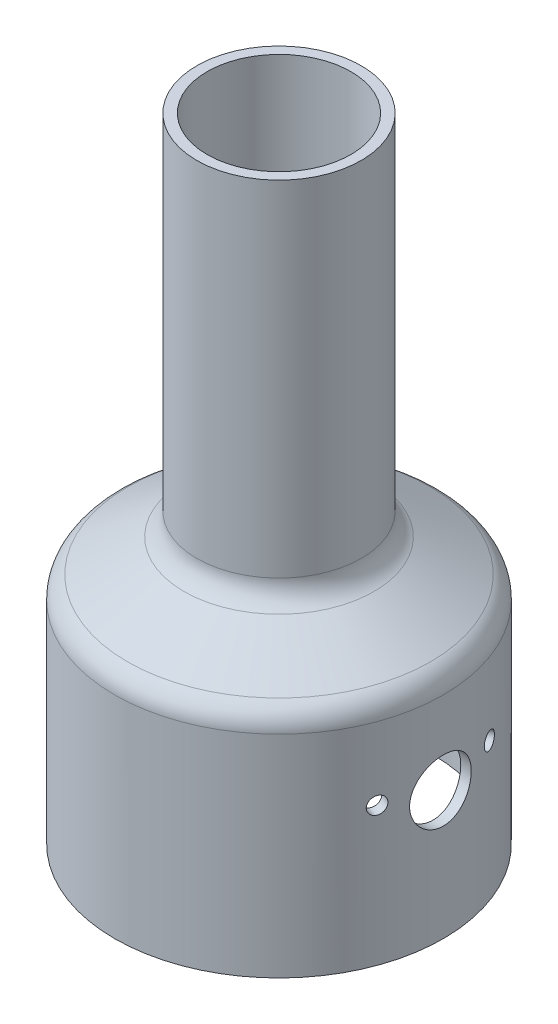
from build123d import *

# Parameters (mm, degrees)
FILLET1_R                       = 5
SHELL1_T                        = -2
CUT_EXTRUDE1_DEPTH              = 132.284070659
CUT_EXTRUDE1_DEPTH_BACK         = 132.284070659
SKETCH6_R                       = 6
M4_TAPPED_HOLE1_D               = 3.3
M4_TAPPED_HOLE1_DEPTH           = 10.1
M4_TAPPED_HOLE1_TIP             = 0.991420021
M4_TAPPED_HOLE1_ON_FACE_2_D     = 3.3
M4_TAPPED_HOLE1_ON_FACE_2_DEPTH = 10.1
M4_TAPPED_HOLE1_ON_FACE_2_TIP   = 0.991420021
M4_TAPPED_HOLE1_ON_FACE_3_D     = 3.3
M4_TAPPED_HOLE1_ON_FACE_3_DEPTH = 10.1
M4_TAPPED_HOLE1_ON_FACE_3_TIP   = 0.991420021
M4_TAPPED_HOLE1_ON_FACE_4_D     = 3.3
M4_TAPPED_HOLE1_ON_FACE_4_DEPTH = 10.1
M4_TAPPED_HOLE1_ON_FACE_4_TIP   = 0.991420021


with BuildPart() as part:
    # Sketch1 → Revolve1 (revolve)
    with BuildSketch(Plane.XY, mode=Mode.PRIVATE) as revolve1_sk:
        Polygon((0, 0), (-32, 0), (-32, 44), (-16, 53.237604307), (-16, 123.237604307), (0, 123.237604307), align=None)
    revolve(revolve1_sk.sketch.rotate(Axis((0, 123.237604307, 0), (0, -1, 0)), 270), axis=Axis((0, 123.237604307, 0), (0, -1, 0)))

    # Fillet1
    fillet1_edges = [part.edges().sort_by_distance(p)[0] for p in [
        (0, 53.237604307, -16),
        (0, 44, -32),
    ]]
    fillet(fillet1_edges, radius=FILLET1_R)

    # Shell1
    shell1_openings = [part.faces().sort_by_distance(p)[0] for p in [
        (0, 123.237604307, 0),
        (0, 0, 0),
    ]]
    offset(amount=SHELL1_T, openings=shell1_openings, kind=Kind.INTERSECTION)

    # Sketch6 → Cut-Extrude1 (cut, two sides: drawn at the far end of the back side and taken through both)
    with BuildSketch(Plane(origin=(0, 0, 0), x_dir=(0, 0, -1), z_dir=(1, 0, 0)).offset(-CUT_EXTRUDE1_DEPTH_BACK)):
        with Locations((0, 25)):
            Circle(SKETCH6_R)
    extrude(amount=CUT_EXTRUDE1_DEPTH + CUT_EXTRUDE1_DEPTH_BACK, mode=Mode.SUBTRACT)

    # M4 Tapped Hole1
    with Locations(Plane(origin=(-30.070163865, 27, -10.944644586), x_dir=(0.342020143326, 0, -0.939692620786), z_dir=(-0.939692620786, 0, -0.342020143326))):
        with Locations((0, 0)):
            Hole(M4_TAPPED_HOLE1_D / 2, depth=M4_TAPPED_HOLE1_DEPTH)
            with Locations((0, 0, -(M4_TAPPED_HOLE1_DEPTH + M4_TAPPED_HOLE1_TIP / 2))):  # 118° drill point
                Cone(0, M4_TAPPED_HOLE1_D / 2, M4_TAPPED_HOLE1_TIP, mode=Mode.SUBTRACT)

    # M4 Tapped Hole1 on face 2
    with Locations(Plane(origin=(-30.070163865, 27, 10.944644586), x_dir=(-0.342019894889, 0, -0.939692711209), z_dir=(-0.939692711209, 0, 0.342019894889))):
        with Locations((0, 0)):
            Hole(M4_TAPPED_HOLE1_ON_FACE_2_D / 2, depth=M4_TAPPED_HOLE1_ON_FACE_2_DEPTH)
            with Locations((0, 0, -(M4_TAPPED_HOLE1_ON_FACE_2_DEPTH + M4_TAPPED_HOLE1_ON_FACE_2_TIP / 2))):  # 118° drill point
                Cone(0, M4_TAPPED_HOLE1_ON_FACE_2_D / 2, M4_TAPPED_HOLE1_ON_FACE_2_TIP, mode=Mode.SUBTRACT)

    # M4 Tapped Hole1 on face 3
    with Locations(Plane(origin=(30.070163865, 27, -10.944644586), x_dir=(0.342019894889, 0, 0.939692711209), z_dir=(0.939692711209, 0, -0.342019894889))):
        with Locations((0, 0)):
            Hole(M4_TAPPED_HOLE1_ON_FACE_3_D / 2, depth=M4_TAPPED_HOLE1_ON_FACE_3_DEPTH)
            with Locations((0, 0, -(M4_TAPPED_HOLE1_ON_FACE_3_DEPTH + M4_TAPPED_HOLE1_ON_FACE_3_TIP / 2))):  # 118° drill point
                Cone(0, M4_TAPPED_HOLE1_ON_FACE_3_D / 2, M4_TAPPED_HOLE1_ON_FACE_3_TIP, mode=Mode.SUBTRACT)

    # M4 Tapped Hole1 on face 4
    with Locations(Plane(origin=(30.070163865, 27, 10.944644586), x_dir=(-0.342019894889, 0, 0.939692711209), z_dir=(0.939692711209, 0, 0.342019894889))):
        with Locations((0, 0)):
            Hole(M4_TAPPED_HOLE1_ON_FACE_4_D / 2, depth=M4_TAPPED_HOLE1_ON_FACE_4_DEPTH)
            with Locations((0, 0, -(M4_TAPPED_HOLE1_ON_FACE_4_DEPTH + M4_TAPPED_HOLE1_ON_FACE_4_TIP / 2))):  # 118° drill point
                Cone(0, M4_TAPPED_HOLE1_ON_FACE_4_D / 2, M4_TAPPED_HOLE1_ON_FACE_4_TIP, mode=Mode.SUBTRACT)


solid = part.part
